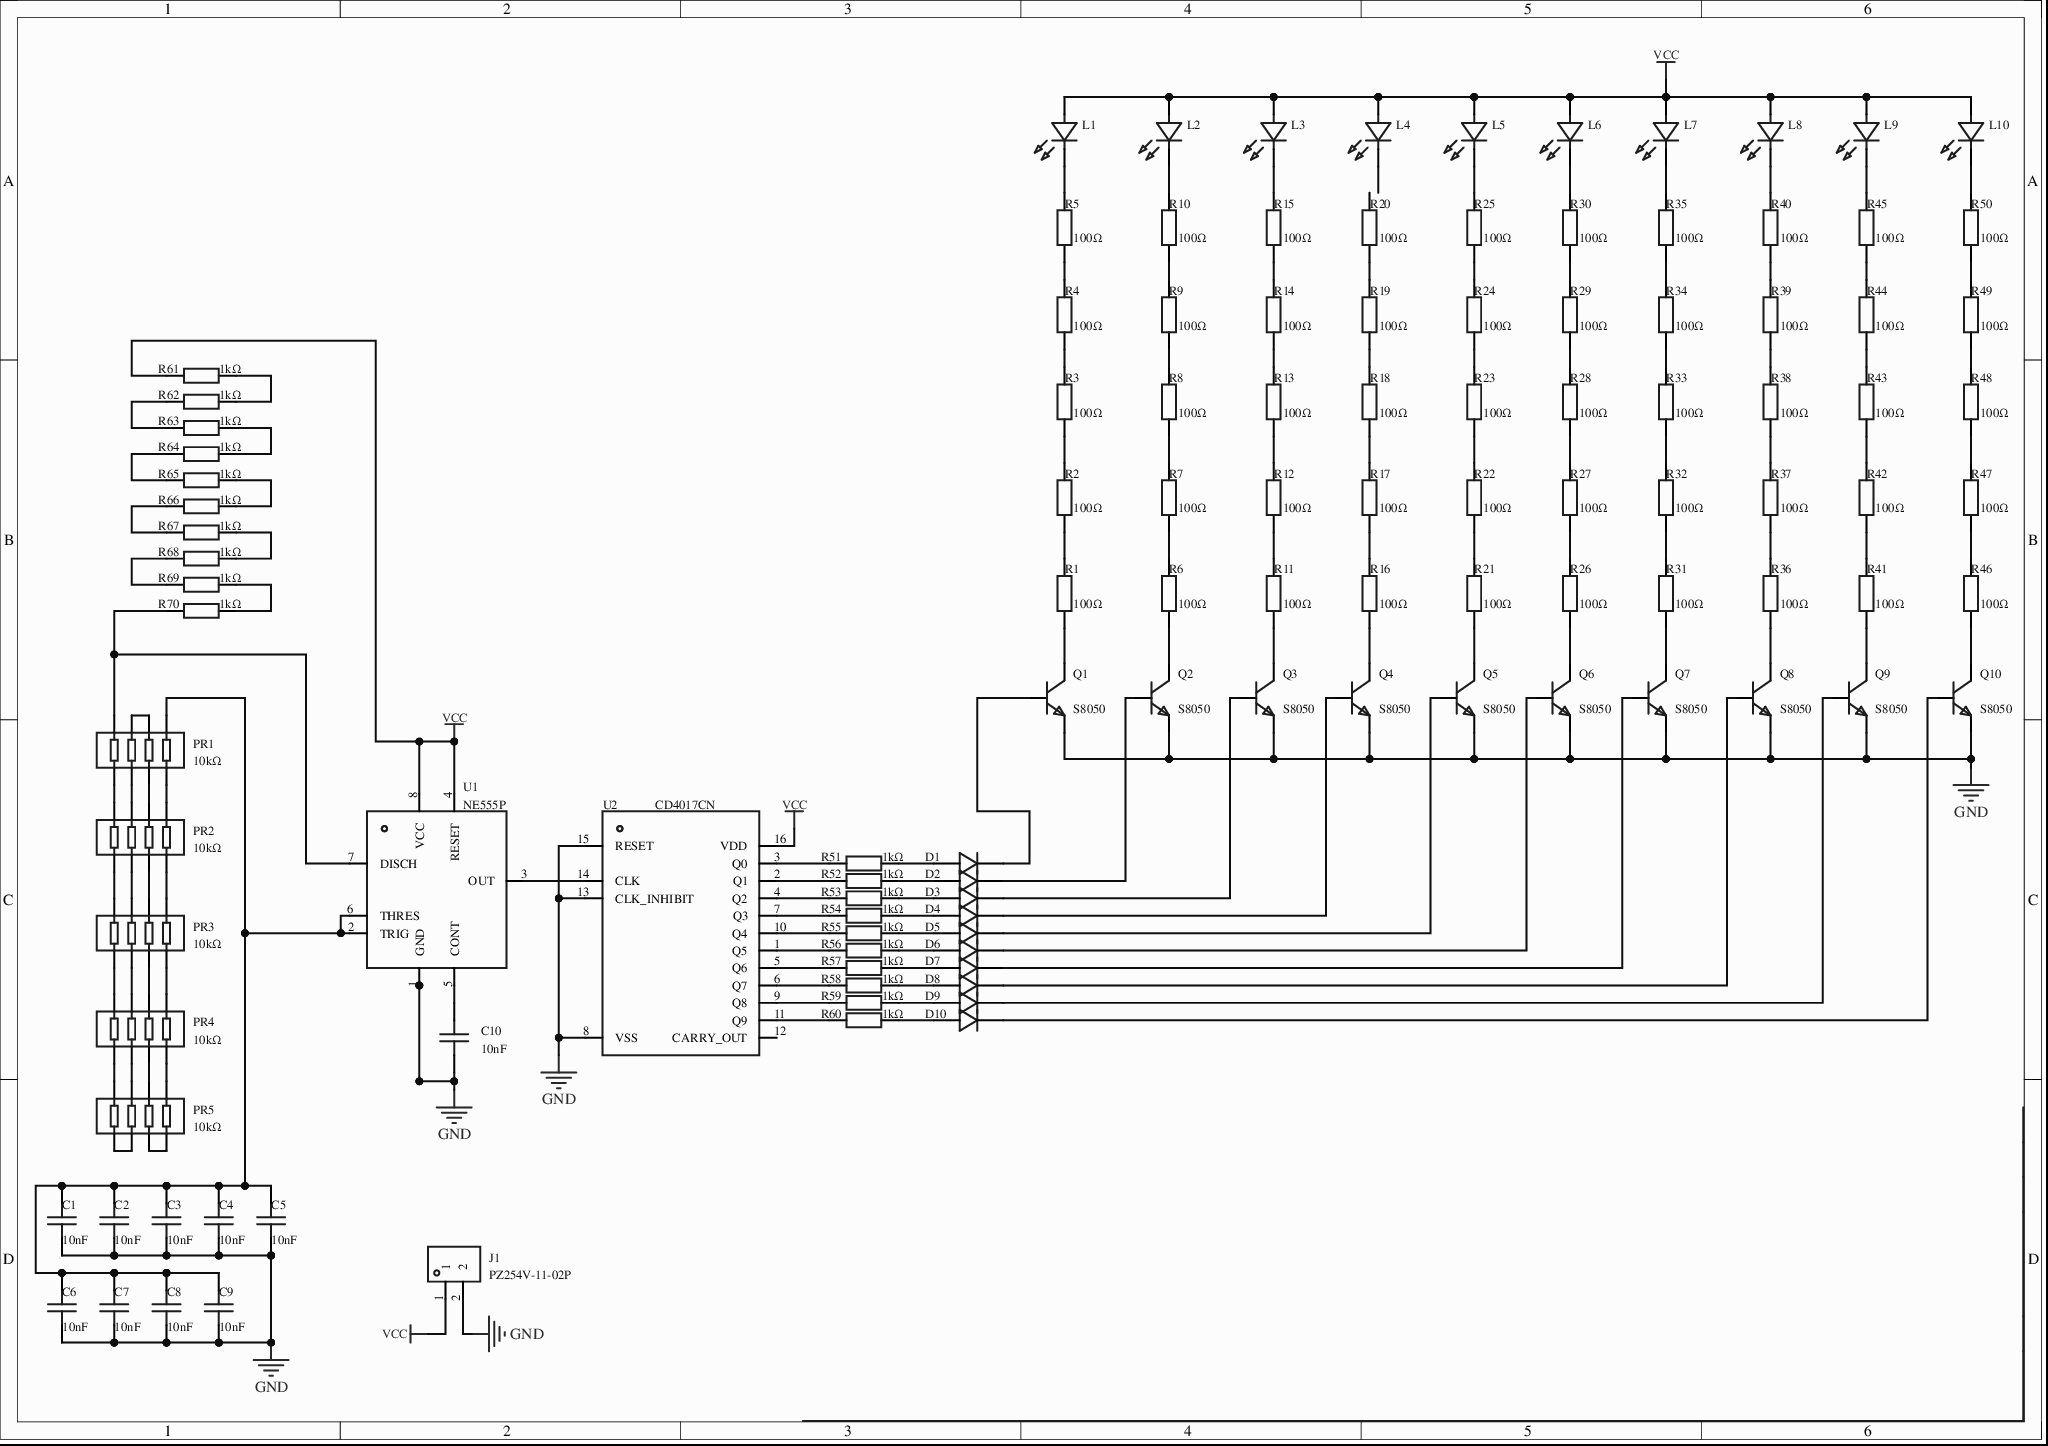
[diagram p0: MISC51982-3.schdoc]
# Altium project MISC51982-2.PrjPcb
1 sheet, 118 parts. Net scope: global (net labels, ports and power ports of the same name join across sheets).
Board file: MISC51982.pcbdoc

## Sheet MISC51982-3.schdoc
size 297 x 209 mm; Version: V1.0; @Project Name: MISC51982; @Page Count: 1; @Update Date: 2026-03-18; @Create Date: 2026-03-18; @Schematic Name: MISC51982; @Page No: 1; @Board Name: MISC51982; @Create Time: 14:32:28; @Update Time: 14:38:12; Size: A4

### Parts
C1  10nF  [CAP-TH_L8.0-W2.8-P5.08-D0.6]
C2  10nF  [CAP-TH_L8.0-W2.8-P5.08-D0.6]
C3  10nF  [CAP-TH_L8.0-W2.8-P5.08-D0.6]
C4  10nF  [CAP-TH_L8.0-W2.8-P5.08-D0.6]
C5  10nF  [CAP-TH_L8.0-W2.8-P5.08-D0.6]
C6  10nF  [CAP-TH_L8.0-W2.8-P5.08-D0.6]
C7  10nF  [CAP-TH_L8.0-W2.8-P5.08-D0.6]
C8  10nF  [CAP-TH_L8.0-W2.8-P5.08-D0.6]
C9  10nF  [CAP-TH_L8.0-W2.8-P5.08-D0.6]
C10  10nF  [CAP-TH_L8.0-W2.8-P5.08-D0.6]
D1  1N4148TR  [DO-35_BD2.0-L4.2-P8.20-D0.5-RD]  (value not drawn)
D2  1N4148TR  [DO-35_BD2.0-L4.2-P8.20-D0.5-RD]  (value not drawn)
D3  1N4148TR  [DO-35_BD2.0-L4.2-P8.20-D0.5-RD]  (value not drawn)
D4  1N4148TR  [DO-35_BD2.0-L4.2-P8.20-D0.5-RD]  (value not drawn)
D5  1N4148TR  [DO-35_BD2.0-L4.2-P8.20-D0.5-RD]  (value not drawn)
D6  1N4148TR  [DO-35_BD2.0-L4.2-P8.20-D0.5-RD]  (value not drawn)
D7  1N4148TR  [DO-35_BD2.0-L4.2-P8.20-D0.5-RD]  (value not drawn)
D8  1N4148TR  [DO-35_BD2.0-L4.2-P8.20-D0.5-RD]  (value not drawn)
D9  1N4148TR  [DO-35_BD2.0-L4.2-P8.20-D0.5-RD]  (value not drawn)
D10  1N4148TR  [DO-35_BD2.0-L4.2-P8.20-D0.5-RD]  (value not drawn)
J1  PZ254V-11-02P  [HDR-TH_2P-P2.54-V-M]
L1  XL-502SURD  [LED-TH_BD5.9-P2.54-RD_RED]  (value not drawn)
L2  XL-502SURD  [LED-TH_BD5.9-P2.54-RD_RED]  (value not drawn)
L3  XL-502SURD  [LED-TH_BD5.9-P2.54-RD_RED]  (value not drawn)
L4  XL-502SURD  [LED-TH_BD5.9-P2.54-RD_RED]  (value not drawn)
L5  XL-502SURD  [LED-TH_BD5.9-P2.54-RD_RED]  (value not drawn)
L6  XL-502SURD  [LED-TH_BD5.9-P2.54-RD_RED]  (value not drawn)
L7  XL-502SURD  [LED-TH_BD5.9-P2.54-RD_RED]  (value not drawn)
L8  XL-502SURD  [LED-TH_BD5.9-P2.54-RD_RED]  (value not drawn)
L9  XL-502SURD  [LED-TH_BD5.9-P2.54-RD_RED]  (value not drawn)
L10  XL-502SURD  [LED-TH_BD5.9-P2.54-RD_RED]  (value not drawn)
PR1  10kΩ  [RES-ARRAY-TH_8P-L20.3-W2.5-P2.54]
PR2  10kΩ  [RES-ARRAY-TH_8P-L20.3-W2.5-P2.54]
PR3  10kΩ  [RES-ARRAY-TH_8P-L20.3-W2.5-P2.54]
PR4  10kΩ  [RES-ARRAY-TH_8P-L20.3-W2.5-P2.54]
PR5  10kΩ  [RES-ARRAY-TH_8P-L20.3-W2.5-P2.54]
Q1  S8050  [TO-92-3_L4.5-W3.5-P1.27-L]
Q2  S8050  [TO-92-3_L4.5-W3.5-P1.27-L]
Q3  S8050  [TO-92-3_L4.5-W3.5-P1.27-L]
Q4  S8050  [TO-92-3_L4.5-W3.5-P1.27-L]
Q5  S8050  [TO-92-3_L4.5-W3.5-P1.27-L]
Q6  S8050  [TO-92-3_L4.5-W3.5-P1.27-L]
Q7  S8050  [TO-92-3_L4.5-W3.5-P1.27-L]
Q8  S8050  [TO-92-3_L4.5-W3.5-P1.27-L]
Q9  S8050  [TO-92-3_L4.5-W3.5-P1.27-L]
Q10  S8050  [TO-92-3_L4.5-W3.5-P1.27-L]
R1  100Ω  [RES-TH_BD2.2-L6.5-P10.50-D0.6]
R2  100Ω  [RES-TH_BD2.2-L6.5-P10.50-D0.6]
R3  100Ω  [RES-TH_BD2.2-L6.5-P10.50-D0.6]
R4  100Ω  [RES-TH_BD2.2-L6.5-P10.50-D0.6]
R5  100Ω  [RES-TH_BD2.2-L6.5-P10.50-D0.6]
R6  100Ω  [RES-TH_BD2.2-L6.5-P10.50-D0.6]
R7  100Ω  [RES-TH_BD2.2-L6.5-P10.50-D0.6]
R8  100Ω  [RES-TH_BD2.2-L6.5-P10.50-D0.6]
R9  100Ω  [RES-TH_BD2.2-L6.5-P10.50-D0.6]
R10  100Ω  [RES-TH_BD2.2-L6.5-P10.50-D0.6]
R11  100Ω  [RES-TH_BD2.2-L6.5-P10.50-D0.6]
R12  100Ω  [RES-TH_BD2.2-L6.5-P10.50-D0.6]
R13  100Ω  [RES-TH_BD2.2-L6.5-P10.50-D0.6]
R14  100Ω  [RES-TH_BD2.2-L6.5-P10.50-D0.6]
R15  100Ω  [RES-TH_BD2.2-L6.5-P10.50-D0.6]
R16  100Ω  [RES-TH_BD2.2-L6.5-P10.50-D0.6]
R17  100Ω  [RES-TH_BD2.2-L6.5-P10.50-D0.6]
R18  100Ω  [RES-TH_BD2.2-L6.5-P10.50-D0.6]
R19  100Ω  [RES-TH_BD2.2-L6.5-P10.50-D0.6]
R20  100Ω  [RES-TH_BD2.2-L6.5-P10.50-D0.6]
R21  100Ω  [RES-TH_BD2.2-L6.5-P10.50-D0.6]
R22  100Ω  [RES-TH_BD2.2-L6.5-P10.50-D0.6]
R23  100Ω  [RES-TH_BD2.2-L6.5-P10.50-D0.6]
R24  100Ω  [RES-TH_BD2.2-L6.5-P10.50-D0.6]
R25  100Ω  [RES-TH_BD2.2-L6.5-P10.50-D0.6]
R26  100Ω  [RES-TH_BD2.2-L6.5-P10.50-D0.6]
R27  100Ω  [RES-TH_BD2.2-L6.5-P10.50-D0.6]
R28  100Ω  [RES-TH_BD2.2-L6.5-P10.50-D0.6]
R29  100Ω  [RES-TH_BD2.2-L6.5-P10.50-D0.6]
R30  100Ω  [RES-TH_BD2.2-L6.5-P10.50-D0.6]
R31  100Ω  [RES-TH_BD2.2-L6.5-P10.50-D0.6]
R32  100Ω  [RES-TH_BD2.2-L6.5-P10.50-D0.6]
R33  100Ω  [RES-TH_BD2.2-L6.5-P10.50-D0.6]
R34  100Ω  [RES-TH_BD2.2-L6.5-P10.50-D0.6]
R35  100Ω  [RES-TH_BD2.2-L6.5-P10.50-D0.6]
R36  100Ω  [RES-TH_BD2.2-L6.5-P10.50-D0.6]
R37  100Ω  [RES-TH_BD2.2-L6.5-P10.50-D0.6]
R38  100Ω  [RES-TH_BD2.2-L6.5-P10.50-D0.6]
R39  100Ω  [RES-TH_BD2.2-L6.5-P10.50-D0.6]
R40  100Ω  [RES-TH_BD2.2-L6.5-P10.50-D0.6]
R41  100Ω  [RES-TH_BD2.2-L6.5-P10.50-D0.6]
R42  100Ω  [RES-TH_BD2.2-L6.5-P10.50-D0.6]
R43  100Ω  [RES-TH_BD2.2-L6.5-P10.50-D0.6]
R44  100Ω  [RES-TH_BD2.2-L6.5-P10.50-D0.6]
R45  100Ω  [RES-TH_BD2.2-L6.5-P10.50-D0.6]
R46  100Ω  [RES-TH_BD2.2-L6.5-P10.50-D0.6]
R47  100Ω  [RES-TH_BD2.2-L6.5-P10.50-D0.6]
R48  100Ω  [RES-TH_BD2.2-L6.5-P10.50-D0.6]
R49  100Ω  [RES-TH_BD2.2-L6.5-P10.50-D0.6]
R50  100Ω  [RES-TH_BD2.2-L6.5-P10.50-D0.6]
R51  1kΩ  [RES-TH_BD2.5-L6.5-P10.50-D0.6]
R52  1kΩ  [RES-TH_BD2.5-L6.5-P10.50-D0.6]
R53  1kΩ  [RES-TH_BD2.5-L6.5-P10.50-D0.6]
R54  1kΩ  [RES-TH_BD2.5-L6.5-P10.50-D0.6]
R55  1kΩ  [RES-TH_BD2.5-L6.5-P10.50-D0.6]
R56  1kΩ  [RES-TH_BD2.5-L6.5-P10.50-D0.6]
R57  1kΩ  [RES-TH_BD2.5-L6.5-P10.50-D0.6]
R58  1kΩ  [RES-TH_BD2.5-L6.5-P10.50-D0.6]
R59  1kΩ  [RES-TH_BD2.5-L6.5-P10.50-D0.6]
R60  1kΩ  [RES-TH_BD2.5-L6.5-P10.50-D0.6]
R61  1kΩ  [RES-TH_BD2.5-L6.5-P10.50-D0.6]
R62  1kΩ  [RES-TH_BD2.5-L6.5-P10.50-D0.6]
R63  1kΩ  [RES-TH_BD2.5-L6.5-P10.50-D0.6]
R64  1kΩ  [RES-TH_BD2.5-L6.5-P10.50-D0.6]
R65  1kΩ  [RES-TH_BD2.5-L6.5-P10.50-D0.6]
R66  1kΩ  [RES-TH_BD2.5-L6.5-P10.50-D0.6]
R67  1kΩ  [RES-TH_BD2.5-L6.5-P10.50-D0.6]
R68  1kΩ  [RES-TH_BD2.5-L6.5-P10.50-D0.6]
R69  1kΩ  [RES-TH_BD2.5-L6.5-P10.50-D0.6]
R70  1kΩ  [RES-TH_BD2.5-L6.5-P10.50-D0.6]
U1  NE555P  [DIP-8_L9.8-W6.6-P2.54-LS7.6-BL]
U2  CD4017CN  [PDIP-16_L19.3-W6.4-P2.54-LS7.94-BL]

### Nets
GND: C1.1 C2.1 C3.1 C4.1 C5.1 C6.1 C7.1 C8.1 C9.1 C10.1 J1.2 Q1.1(E) Q2.1(E) Q3.1(E) Q4.1(E) Q5.1(E) Q6.1(E) Q7.1(E) Q8.1(E) Q9.1(E) Q10.1(E) U1.1(GND) U2.8(VSS) U2.13(CLK_INHIBIT) U2.15(RESET)
VCC: J1.1 L1.2(A) L2.2(A) L3.2(A) L4.2(A) L5.2(A) L6.2(A) L7.2(A) L8.2(A) L9.2(A) L10.2(A) R61.1 U1.4(RESET) U1.8(VCC) U2.16(VDD)
NetC1_2: C1.2 C2.2 C3.2 C4.2 C5.2 C6.2 C7.2 C8.2 C9.2 PR1.5 U1.2(TRIG) U1.6(THRES)
NetC10_2: C10.2 U1.5(CONT)
NetD1_1: D1.1(C) Q1.2(B)
NetD1_2: D1.2(A) R51.2
NetD2_1: D2.1(C) Q2.2(B)
NetD2_2: D2.2(A) R52.2
NetD3_1: D3.1(C) Q3.2(B)
NetD3_2: D3.2(A) R53.2
NetD4_1: D4.1(C) Q4.2(B)
NetD4_2: D4.2(A) R54.2
NetD5_1: D5.1(C) Q5.2(B)
NetD5_2: D5.2(A) R55.2
NetD6_1: D6.1(C) Q6.2(B)
NetD6_2: D6.2(A) R56.2
NetD7_1: D7.1(C) Q7.2(B)
NetD7_2: D7.2(A) R57.2
NetD8_1: D8.1(C) Q8.2(B)
NetD8_2: D8.2(A) R58.2
NetD9_1: D9.1(C) Q9.2(B)
NetD9_2: D9.2(A) R59.2
NetD10_1: D10.1(C) Q10.2(B)
NetD10_2: D10.2(A) R60.2
NetL1_1: L1.1(K) R5.2
NetL2_1: L2.1(K) R10.2
NetL3_1: L3.1(K) R15.2
NetL5_1: L5.1(K) R25.2
NetL6_1: L6.1(K) R30.2
NetL7_1: L7.1(K) R35.2
NetL8_1: L8.1(K) R40.2
NetL9_1: L9.1(K) R45.2
NetL10_1: L10.1(K) R50.2
NetPR1_1: PR1.1 PR2.8
NetPR1_2: PR1.2 PR2.7
NetPR1_3: PR1.3 PR2.6
NetPR1_4: PR1.4 PR2.5
NetPR1_6: PR1.6 PR1.7
NetPR1_8: PR1.8 R70.1 U1.7(DISCH)
NetPR2_1: PR2.1 PR3.8
NetPR2_2: PR2.2 PR3.7
NetPR2_3: PR2.3 PR3.6
NetPR2_4: PR2.4 PR3.5
NetPR3_1: PR3.1 PR4.8
NetPR3_2: PR3.2 PR4.7
NetPR3_3: PR3.3 PR4.6
NetPR3_4: PR3.4 PR4.5
NetPR4_1: PR4.1 PR5.8
NetPR4_2: PR4.2 PR5.7
NetPR4_3: PR4.3 PR5.6
NetPR4_4: PR4.4 PR5.5
NetPR5_1: PR5.1 PR5.2
NetPR5_3: PR5.3 PR5.4
NetQ1_3: Q1.3(C) R1.1
NetQ2_3: Q2.3(C) R6.1
NetQ3_3: Q3.3(C) R11.1
NetQ4_3: Q4.3(C) R16.1
NetQ5_3: Q5.3(C) R21.1
NetQ6_3: Q6.3(C) R26.1
NetQ7_3: Q7.3(C) R31.1
NetQ8_3: Q8.3(C) R36.1
NetQ9_3: Q9.3(C) R41.1
NetQ10_3: Q10.3(C) R46.1
NetR1_2: R1.2 R2.1
NetR2_2: R2.2 R3.1
NetR3_2: R3.2 R4.1
NetR4_2: R4.2 R5.1
NetR6_2: R6.2 R7.1
NetR7_2: R7.2 R8.1
NetR8_2: R8.2 R9.1
NetR9_2: R9.2 R10.1
NetR11_2: R11.2 R12.1
NetR12_2: R12.2 R13.1
NetR13_2: R13.2 R14.1
NetR14_2: R14.2 R15.1
NetR16_2: R16.2 R17.1
NetR17_2: R17.2 R18.1
NetR18_2: R18.2 R19.1
NetR19_2: R19.2 R20.1
NetR21_2: R21.2 R22.1
NetR22_2: R22.2 R23.1
NetR23_2: R23.2 R24.1
NetR24_2: R24.2 R25.1
NetR26_2: R26.2 R27.1
NetR27_2: R27.2 R28.1
NetR28_2: R28.2 R29.1
NetR29_2: R29.2 R30.1
NetR31_2: R31.2 R32.1
NetR32_2: R32.2 R33.1
NetR33_2: R33.2 R34.1
NetR34_2: R34.2 R35.1
NetR36_2: R36.2 R37.1
NetR37_2: R37.2 R38.1
NetR38_2: R38.2 R39.1
NetR39_2: R39.2 R40.1
NetR41_2: R41.2 R42.1
NetR42_2: R42.2 R43.1
NetR43_2: R43.2 R44.1
NetR44_2: R44.2 R45.1
NetR46_2: R46.2 R47.1
NetR47_2: R47.2 R48.1
NetR48_2: R48.2 R49.1
NetR49_2: R49.2 R50.1
NetR51_1: R51.1 U2.3(Q0)
NetR52_1: R52.1 U2.2(Q1)
NetR53_1: R53.1 U2.4(Q2)
NetR54_1: R54.1 U2.7(Q3)
NetR55_1: R55.1 U2.10(Q4)
NetR56_1: R56.1 U2.1(Q5)
NetR57_1: R57.1 U2.5(Q6)
NetR58_1: R58.1 U2.6(Q7)
NetR59_1: R59.1 U2.9(Q8)
NetR60_1: R60.1 U2.11(Q9)
NetR61_2: R61.2 R62.2
NetR62_1: R62.1 R63.1
NetR63_2: R63.2 R64.2
NetR64_1: R64.1 R65.1
NetR65_2: R65.2 R66.2
NetR66_1: R66.1 R67.1
NetR67_2: R67.2 R68.2
NetR68_1: R68.1 R69.1
NetR69_2: R69.2 R70.2
NetU1_3: U1.3(OUT) U2.14(CLK)

Not connected (* = marked no-connect by the designer): L4 1(K); R20 2; U2 12(CARRY_OUT)

### Library data of the parts
C1-C10 = CC3A103MC1IEF48C30MF: 容值:10nF;精度:±20%;额定电压:1kV;温度系数:Y5V;; Manufacturer: Dersonic(德尔创); AddInBom: yes; Tolerance: ±20%; Voltage Rating: 1kV; Pin Spacing: 5.08mm; Temperature Coefficient: Y5V; Body Thickness: 2.8mm; ModelId: adc2ba9dad3c618c; ModelTransform: 0,0,0,0,0,0,0,0,0; Device: CC3A103MC1IEF48C30MF; Symbol: CC3A103MC1IEF48C30MF; FootprintName: CAP-TH_L8.0-W2.8-P5.08-D0.6; LCSC Part Name: 10nF ±20% 1kV; SupplierPart: C263209; ManufacturerPart: CC3A103MC1IEF48C30MF; Supplier Footprint: 插件,P=5.08mm; JLCPCB Part Class: 扩展库; Datasheet: https://item.szlcsc.com/datasheet/CC3A103MC1IEF48C30MF/254325.html; Supplier: LCSC; ConvertToPcb: yes; Value: 10nF; Diameter: 8mm; ModelName: CAP-TH_L8.0-W2.8-P5.08-D0.6
D1-D10 = 1N4148TR_C84410: 二极管配置:-;正向压降(Vf):1V@10mA;直流反向耐压(Vr):100V;整流电流:200mA;反向恢复时间(Trr):4ns;; Manufacturer: onsemi(安森美); AddInBom: yes; Voltage - DC Reverse(Vr): 100V; Current - Rectified: 200mA; Pd - Power Dissipation: 500mW; Reverse Leakage Current (Ir): 5uA@75V; Reverse Recovery Time (trr): 4ns; Operating Junction Temperature Range: -55℃~+175℃@(Tj); Non-Repetitive Peak Forward Surge Current: 4A; ModelId: 6e6fa891745c42b796728c269d94cdcf; ModelName: DO-35_D1.9-L3.9-P8.2; ModelTransform: 342.519,74.82103,0,0,0,0,-0.197,1.181,-137.795; Device: 1N4148TR_C84410; Symbol: 1N4148TR; FootprintName: DO-35_BD2.0-L4.2-P8.20-D0.5-RD; LCSC Part Name: 1N4148TR; SupplierPart: C84410; ManufacturerPart: 1N4148TR; Supplier Footprint: DO-35; JLCPCB Part Class: 扩展库; Datasheet: https://item.szlcsc.com/datasheet/1N4148TR/85580.html; Supplier: LCSC; ConvertToPcb: yes; Diode Configuration: -; Voltage - Forward(Vf@If): 1V@10mA
J1 = PZ254V-11-02P: 插针结构:1x2P;间距:2.54mm;行距:-;圆针/方针:方针;安装方式:直插;排数:单排;总PIN位数:2P;额定电流:3A;额定电压:250V;配合针长度:6mm;塑高:2.5mm;端接针长度:3mm;触头材质:黄铜;触头镀层:-;工作温度:-40℃~+105℃;颜色:黑色;; Manufacturer: XFCN(兴飞); AddInBom: yes; Pin Structure: 1x2P; Pitch: 2.54mm; Circluar Pins/Square Pins: 方针; Current Rating: 3A; Voltage Rating (Max): 250V; ModelId: e35305ec3aa84b66b849f914b715e73f; ModelName: HDR2.54-M-LI-1X2P; ModelTransform: 200,100,0,0,0,0,0,0,-118.11; Device: PZ254V-11-02P; Symbol: PZ254V-11-02P; FootprintName: HDR-TH_2P-P2.54-V-M; LCSC Part Name: 1x2P 间距:2.54mm 方针 直插; SupplierPart: C492401; ManufacturerPart: PZ254V-11-02P; Supplier Footprint: 插件,P=2.54mm; JLCPCB Part Class: 扩展库; Datasheet: https://item.szlcsc.com/datasheet/PZ254V-11-02P/502957.html; Supplier: LCSC; ConvertToPcb: yes; Row Spacing: -; Mounting Type: 直插; Number of Rows: 单排; Number of Pins: 2P; Length of Mating Pin: 6mm; Insulation Height: 2.5mm; Length of End Connection Pin: 3mm; Contact Material: 黄铜; Contact Plating: -; Operating Temperature: -40℃~+105℃; Color: 黑色
L1-L10 = XL-502SURD: 灯头类型:5mm圆形灯头;发光颜色:红色;正向压降(Vf):2.4V;功率:70mW;正向电流:20mA;波长:615nm~625nm;二极管配置:-;透镜颜色:红色透镜;色温:-;发光强度:300mcd;发光角度:35°;载带方式:-;工作温度:-25℃~+85℃;; Manufacturer: XINGLIGHT(成兴光); AddInBom: yes; Illumination Color: 红色; Voltage - Forward(Vf): 2.4V; Power(Watts): 70mW; Forward Current: 20mA; Peak Wavelength: 654nm; Lens Color: 红色透镜; Luminous Intensity: 300mcd; Viewing Angle: 35°; ModelId: fe9cea1bdf7642cd8d9a5077ed0e2b58; ModelTransform: 211.96686,228.01584,0,0,0,0,7.874,0,-137.795; Device: XL-502SURD; Symbol: XL-502SURD; FootprintName: LED-TH_BD5.9-P2.54-RD_RED; LCSC Part Name: 5mm圆形灯头 红色; SupplierPart: C2895492; ManufacturerPart: XL-502SURD; Supplier Footprint: 插件,D=5mm; JLCPCB Part Class: 扩展库; Datasheet: https://item.szlcsc.com/datasheet/XL-502SURD/3136207.html; Supplier: LCSC; ConvertToPcb: yes; Lamp Holder Type: 5mm圆形灯头; Wavelength - Dominant: 615nm~625nm; Diode Configuration: -; Color Temperature: -; Mounting Style: -; Operating Temperature: -25℃~+85℃; ModelName: LED-TH_BD5.9-P2.54-RD_RED
PR1-PR5 = 4608X-102-103LF: 电阻器数:4;阻值:10kΩ;精度:±2%;单个元件功率:300mW;温度系数:±100ppm/℃;; Manufacturer: BOURNS; AddInBom: yes; Number of Resistors: 4; Tolerance: ±2%; Power(Watts): 300mW; ModelId: 1fcaf8e202754517bf5022a866f874ea; ModelTransform: 798.02982,98.031,0,0,0,0,0,0,-133.858; Device: 4608X-102-103LF; Symbol: 4608X-102-103LF; FootprintName: RES-ARRAY-TH_8P-L20.3-W2.5-P2.54; LCSC Part Name: 10kΩ ±2%; SupplierPart: C840662; ManufacturerPart: 4608X-102-103LF; Supplier Footprint: SIP-8; JLCPCB Part Class: 扩展库; Datasheet: https://item.szlcsc.com/datasheet/4608X-102-103LF/897114.html; Supplier: LCSC; ConvertToPcb: yes; Value: 10kΩ; Temperature Coefficient: ±100ppm/℃; Number of Pins: 8; ModelName: RES-ARRAY-TH_8P-L20.3-W2.5-P2.54
Q1-Q10 = S8050_C2931492: 晶体管类型:NPN;集电极电流(Ic):500mA;集射极击穿电压(Vceo):25V;耗散功率(Pd):625mW;直流电流增益(hFE):160@50mA,1V;; Manufacturer: JSMSEMI(杰盛微); AddInBom: yes; type: NPN; Current - Collector(Ic): 500mA; Collector - Emitter Voltage VCEO: 25V; Pd - Power Dissipation: 625mW; Transition frequency(fT): 150MHz; Current - Collector Cutoff: 100nA; Vce Saturation(VCE(sat)): 600mV@500mA,50mA; Emitter-Base Voltage(Vebo): 5V; ModelId: 3c10f07c6cc72ff5; ModelTransform: 0,0,0,0,0,0,0,0,0; Device: S8050_C2931492; Symbol: S8050_C2931492; FootprintName: TO-92-3_L4.5-W3.5-P1.27-L; LCSC Part Name: NPN 电流:500mA 电压:25V; SupplierPart: C2931492; ManufacturerPart: S8050; Supplier Footprint: TO-92; JLCPCB Part Class: 扩展库; Datasheet: https://item.szlcsc.com/datasheet/S8050/3272796.html; Supplier: LCSC; ConvertToPcb: yes; DC Current Gain: 160@50mA,1V; ModelName: TO-92-3_L4.5-W3.5-P1.27-L
R1-R50 = MFR0W4F1000A50: 电阻类型:金属膜电阻;阻值:100Ω;精度:±1%;功率:250mW;温度系数:±50ppm/℃;; Manufacturer: UNI-ROYAL(厚声); AddInBom: yes; Tolerance: ±1%; Voltage-Supply(Max): 250V; Power(Watts): 250mW; ModelId: 094322567e2be2d4; ModelTransform: 0,0,0,0,0,0,0,0,0; Device: MFR0W4F1000A50; Symbol: MFR0W4F1000A50; FootprintName: RES-TH_BD2.2-L6.5-P10.50-D0.6; LCSC Part Name: 100Ω ±1% 250mW 金属膜电阻 铜脚，圆柱状直插; SupplierPart: C57438; ManufacturerPart: MFR0W4F1000A50; Supplier Footprint: 插件,D2.2xL6.5mm; JLCPCB Part Class: 扩展库; Datasheet: https://atta.szlcsc.com/upload/public/pdf/source/20191012/C436293_8820AA14BC71FA35E551C06C441482A0.pdf; Supplier: LCSC; ConvertToPcb: yes; Type: 金属膜电阻; Value: 100Ω; Temperature Coefficient: ±50ppm/℃; ModelName: RES-TH_BD2.2-L6.5-P10.50-D0.6
R51-R70 = MFR0W4F1001A50: 电阻类型:金属膜电阻;阻值:1kΩ;精度:±1%;功率:250mW;温度系数:±50ppm/℃;; Manufacturer: UNI-ROYAL(厚声); AddInBom: yes; Tolerance: ±1%; Voltage-Supply(Max): 250V; Power(Watts): 250mW; ModelId: 8e6c7ee8323443d1ab8f0504b6353c8c; ModelName: RES-TH_D2.3-L6.5-P10.50; ModelTransform: 431.1015,91.3384,0,0,0,0,0.197,0,-137.795; Device: MFR0W4F1001A50; Symbol: MFR0W4F1001A50; FootprintName: RES-TH_BD2.5-L6.5-P10.50-D0.6; LCSC Part Name: 1kΩ ±1% 250mW 金属膜电阻 铜脚，圆柱状直插; SupplierPart: C57435; ManufacturerPart: MFR0W4F1001A50; Supplier Footprint: 插件,D2.2xL6.5mm; JLCPCB Part Class: 扩展库; Datasheet: https://atta.szlcsc.com/upload/public/pdf/source/20191012/C436293_8820AA14BC71FA35E551C06C441482A0.pdf; Supplier: LCSC; ConvertToPcb: yes; Type: 金属膜电阻; Value: 1kΩ; Temperature Coefficient: ±50ppm/℃
U1 = NE555P: 这些器件是精密定时电路，能够产生精确的时间延迟或振荡。在延时或单稳态工作模式下，定时时间间隔由单个外部电阻和电容网络控制。在无稳态工作模式下，频率和占空比可通过两个外部电阻和一个外部电容分别控制; Manufacturer: TI(德州仪器); AddInBom: yes; ModelId: db2af726fcec488f8bf8e467aca974b3; ModelName: DIP-8_L9.8-W6.6-H3.5-LS7.62-P2.54; ModelTransform: 385.826,311.8104,0,0,0,0,-1.693,0,-137.795; Device: NE555P; Symbol: NE555P; FootprintName: DIP-8_L9.8-W6.6-P2.54-LS7.6-BL; LCSC Part Name: NE555P; SupplierPart: C46749; ManufacturerPart: NE555P; Supplier Footprint: DIP-8; JLCPCB Part Class: Extended Part; Datasheet: https://www.ti.com/cn/lit/gpn/ne555; Supplier: LCSC; ConvertToPcb: yes
U2 = CD4017CN: CD4017BE升级替代料，建议试样，5 阶 Johnson 译码计数器; Manufacturer: HGSEMI(华冠); AddInBom: yes; ModelId: 96ff5d01b3074dd183bcbc4cd00a63de; ModelTransform: 759.841,322.44,0,0,0,0,0,0,-137.795; Device: CD4017CN; Symbol: CD4017CN; FootprintName: PDIP-16_L19.3-W6.4-P2.54-LS7.94-BL; LCSC Part Name: CD4017CN; SupplierPart: C20613262; ManufacturerPart: CD4017CN; Supplier Footprint: DIP-16; JLCPCB Part Class: 扩展库; Datasheet: https://atta.szlcsc.com/upload/public/pdf/source/20240202/A11F5FEC5EC92025B33B6A151300674C.pdf; Supplier: LCSC; ConvertToPcb: yes; ModelName: PDIP-16_L19.3-W6.4-P2.54-LS7.94-BL